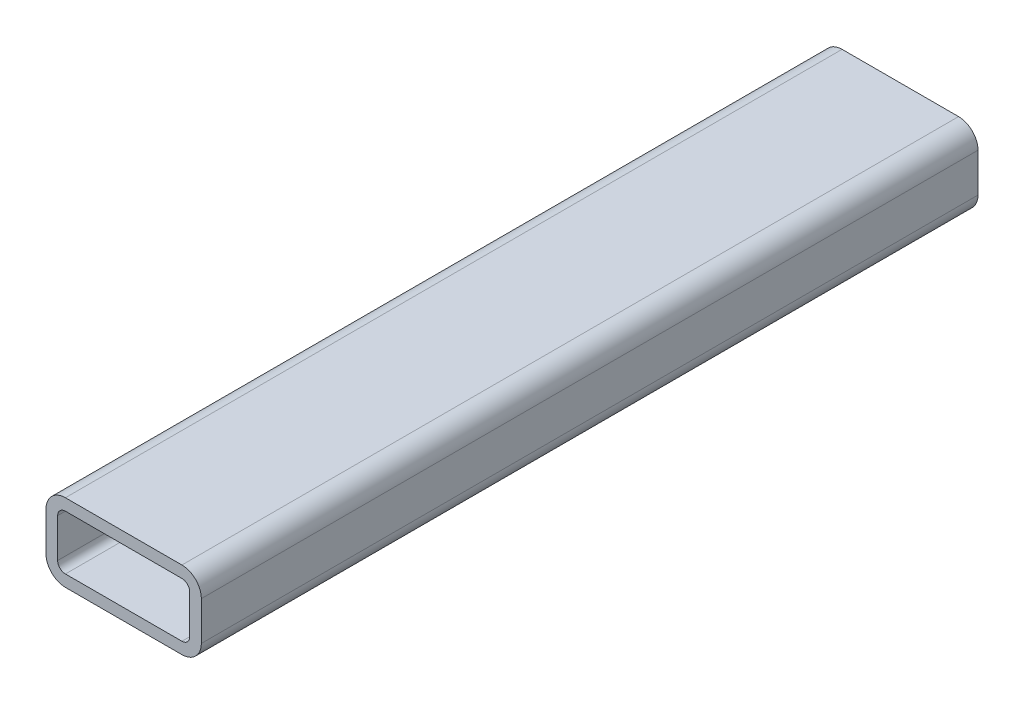
SolidWorks part; units mm, degrees
material "AISI 1045 钢，冷拔"
ref_plane "Front Plane" through (0, 0, 0) normal (0, 0, 1) x (1, 0, 0)
ref_plane "Top Plane" through (0, 0, 0) normal (0, 1, 0) x (1, 0, 0)
ref_plane "Right Plane" through (0, 0, 0) normal (1, 0, 0) x (0, 0, -1)
sketch "Sketch1" plane through (0, 0, 0) normal (0, 0, 1) x (1, 0, 0)
  line L0 (5, 17) -> (35, 17)
  line L1 (5, 0) -> (35, 0)
  line L2 (0, 5) -> (0, 15)
  line L3 (5, 20) -> (35, 20)
  line L4 (40, 5) -> (40, 15)
  line L5 (37, 5) -> (37, 15)
  line L6 (5, 3) -> (35, 3)
  line L7 (3, 5) -> (3, 15)
  arc A0 (35, 0) -> (40, 5) centre (35, 5) ccw
  arc A1 (0, 15) -> (5, 20) centre (5, 15) cw
  arc A2 (35, 20) -> (40, 15) centre (35, 15) cw
  arc A3 (5, 0) -> (0, 5) centre (5, 5) cw
  arc A4 (35, 17) -> (37, 15) centre (35, 15) cw
  arc A5 (35, 3) -> (37, 5) centre (35, 5) ccw
  arc A6 (5, 3) -> (3, 5) centre (5, 5) cw
  arc A7 (3, 15) -> (5, 17) centre (5, 15) cw
  point P7 (40, 0)
  point P10 (0, 20)
  point P15 (0, 0)
  dimension "D3" = 5
  dimension "D1" = 20
  dimension "D2" = 40
  dimension "D4" = 3
extrude "Boss-Extrude1" add sketch "Sketch1" along normal blind 200
